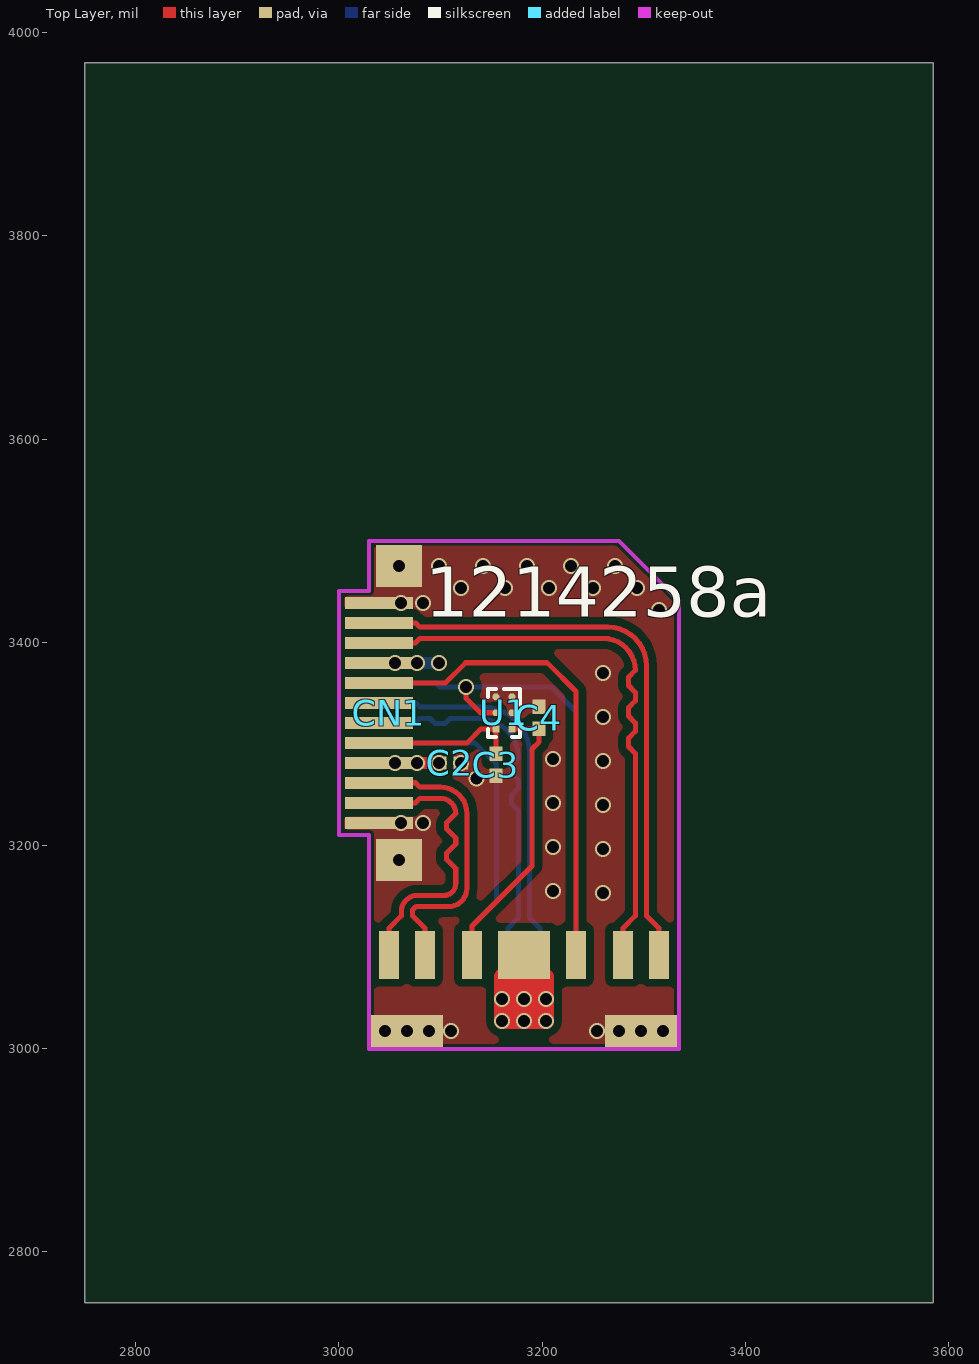
[diagram p0: Top Layer view]
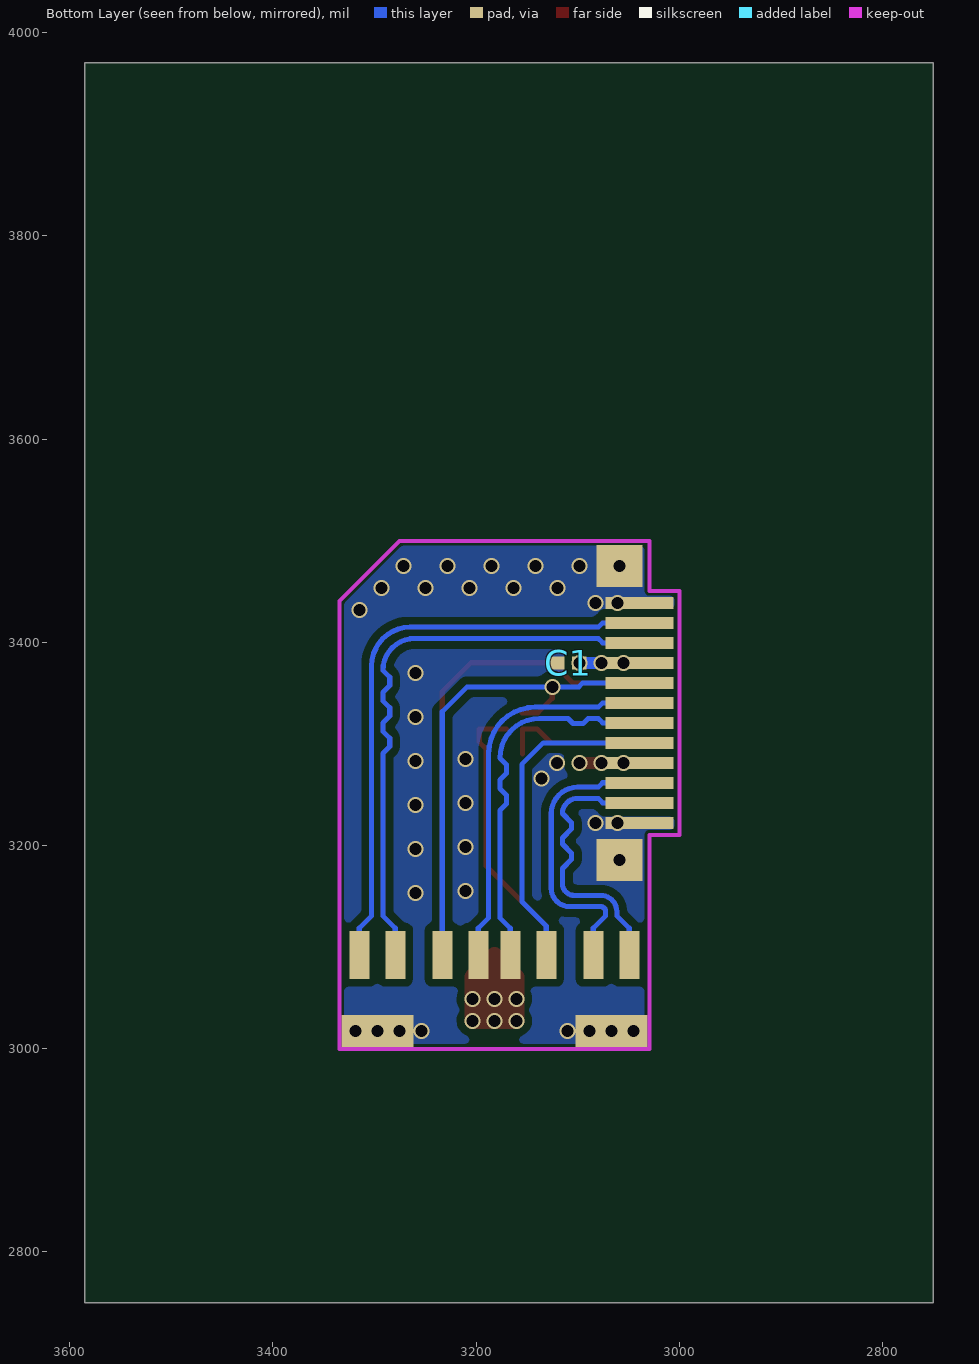
[diagram p1: Bottom Layer view, seen from below]
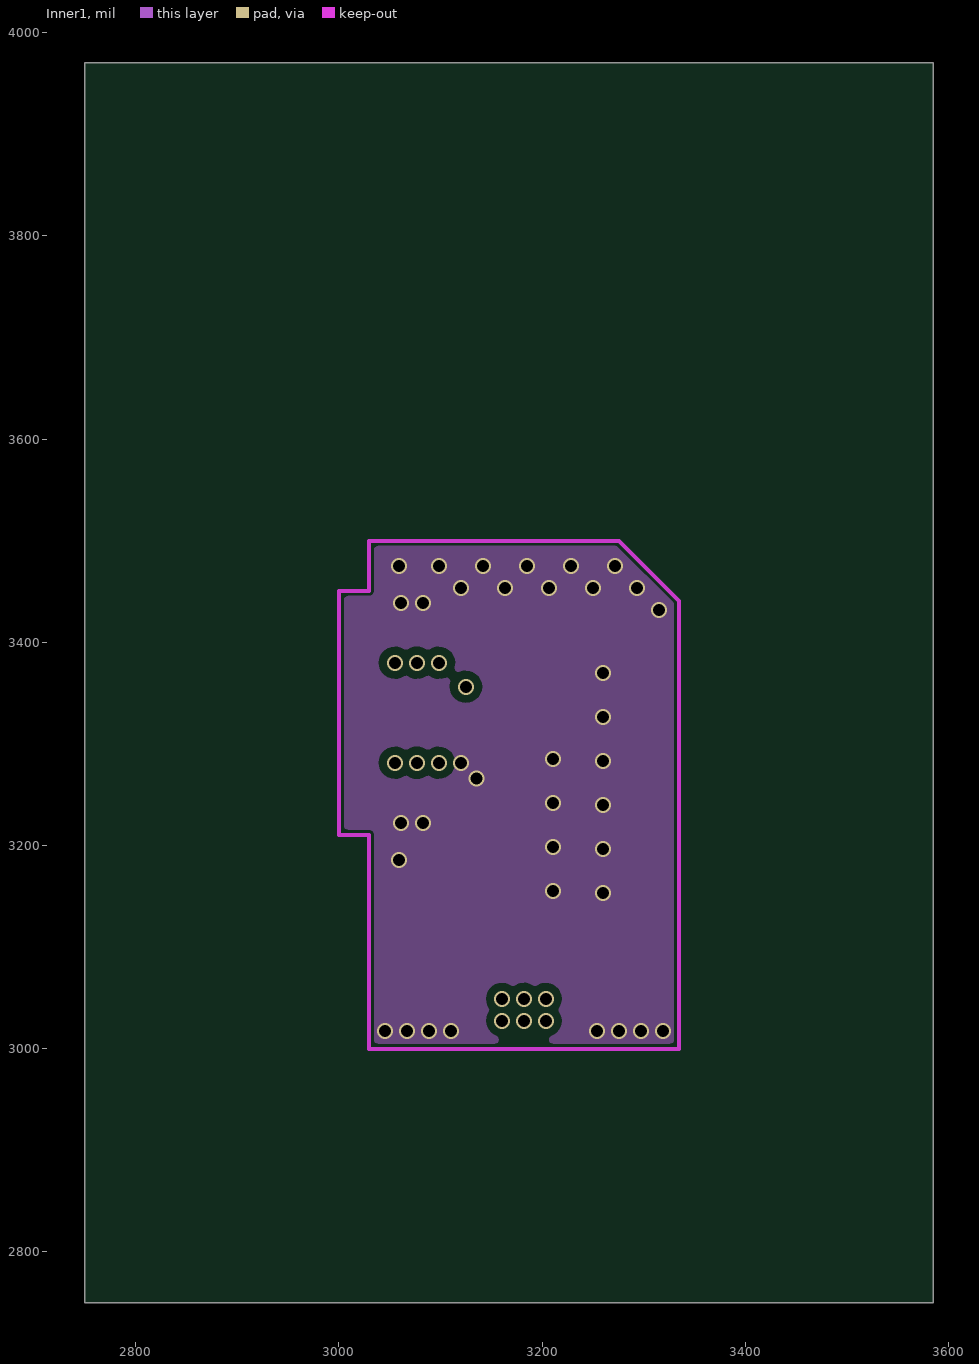
[diagram p2: Inner1]
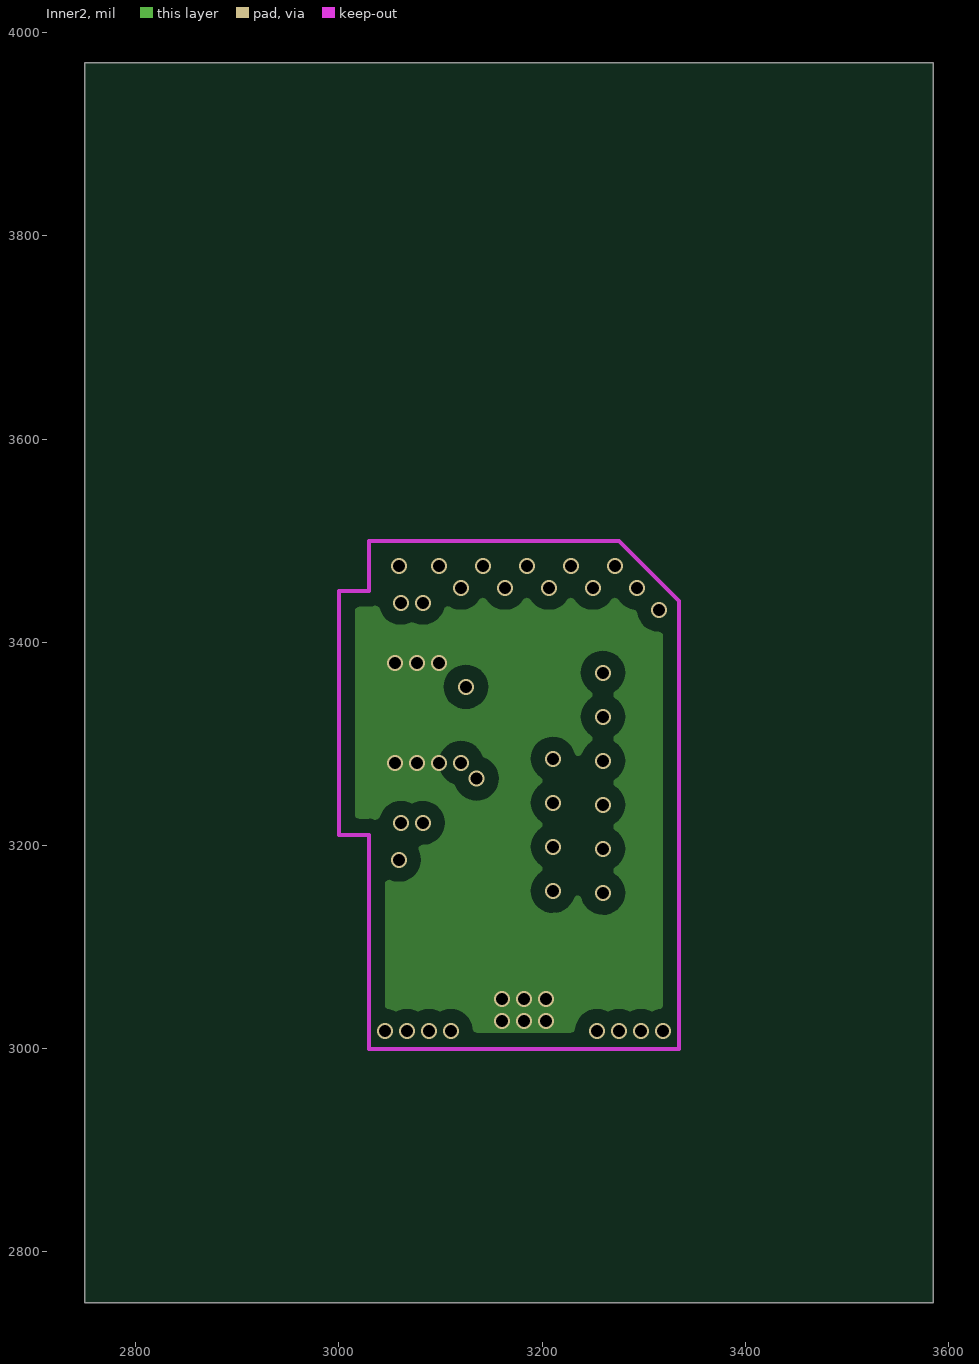
[diagram p3: Inner2]
# Altium PCB MISC82881.pcbdoc
Units mil, origin at the board's own origin, x right, y up, seen from the top; angles counter-clockwise.
Board outline 835 x 1220.35 mil, 4 copper layers (Top Layer, Inner1, Inner2, Bottom Layer), stack 30.706 mil thick; 6 components, 17 nets, 61 pads, 50 vias.

## Layer stack, top to bottom
Top Solder Mask Layer: solder mask 0.394, Dk 0
Top Layer: signal copper 1.378
Dielectric1: surface 8.398, 7628 RC49% 8.6mil, Dk 0
Inner1: signal copper 1.378
Dielectric2: surface 8.398, 1.1mm H/HOZ 含铜, Dk 0
Inner2: signal copper 1.378
Dielectric3: surface 8.398, 7628 RC49% 8.6mil, Dk 0
Bottom Layer: signal copper 1.378
Bottom Solder Mask Layer: solder mask 0.394, Dk 0

## Board outline
3585,2750 2750,2750 2750,3970.35 3585,3970.35

## Design rules (kind name [scope] priority, off if disabled: settings)
BoardOutlineClearance copperThickness2oz_1 [All] p2 off: genericclearance=7.99 ignorepadtopadclearanceinfootprint=FALSE except(0: Arc-SplitContinuation Track-SplitContinuation SMDPad-SplitContinuation THPad-SplitContinuation Via-SplitContinuation Fill-SplitContinuation Region-SplitContinuation Poly-SplitContinuation Text-SplitContinuation Hole-SplitContinuation; 5.98: SMDPad-CutoutEdge THPad-CutoutEdge Via-CutoutEdge Fill-CutoutEdge Region-CutoutEdge Text-CutoutEdge Hole-CutoutEdge; 11.81: Arc-OutlineEdge Track-OutlineEdge SMDPad-OutlineEdge THPad-OutlineEdge Via-OutlineEdge Fill-OutlineEdge Region-OutlineEdge Text-OutlineEdge Hole-OutlineEdge Arc-CutoutEdge Track-CutoutEdge; 13.78: Poly-OutlineEdge Poly-CutoutEdge)
BoardOutlineClearance Plane_innerPlane_1 [All] p4 off: genericclearance=4.02 ignorepadtopadclearanceinfootprint=FALSE except(0: Arc-SplitContinuation Track-SplitContinuation SMDPad-SplitContinuation THPad-SplitContinuation Via-SplitContinuation Fill-SplitContinuation Region-SplitContinuation Poly-SplitContinuation Text-SplitContinuation Hole-SplitContinuation; 5.98: SMDPad-CutoutEdge THPad-CutoutEdge Via-CutoutEdge Fill-CutoutEdge Region-CutoutEdge Text-CutoutEdge Hole-CutoutEdge; 10: Poly-OutlineEdge Poly-CutoutEdge; 11.81: Arc-OutlineEdge Track-OutlineEdge SMDPad-OutlineEdge THPad-OutlineEdge Via-OutlineEdge Fill-OutlineEdge Region-OutlineEdge Text-OutlineEdge Hole-OutlineEdge Arc-CutoutEdge Track-CutoutEdge)
BoardOutlineClearance Copper_copperRegion_1 [All] p6 off: genericclearance=4.02 ignorepadtopadclearanceinfootprint=FALSE except(0: Arc-SplitContinuation Track-SplitContinuation SMDPad-SplitContinuation THPad-SplitContinuation Via-SplitContinuation Fill-SplitContinuation Region-SplitContinuation Poly-SplitContinuation Text-SplitContinuation Hole-SplitContinuation; 5.98: SMDPad-CutoutEdge THPad-CutoutEdge Via-CutoutEdge Fill-CutoutEdge Region-CutoutEdge Text-CutoutEdge Hole-CutoutEdge; 11.81: Arc-OutlineEdge Track-OutlineEdge SMDPad-OutlineEdge THPad-OutlineEdge Via-OutlineEdge Fill-OutlineEdge Region-OutlineEdge Text-OutlineEdge Hole-OutlineEdge Arc-CutoutEdge Track-CutoutEdge; 15.75: Poly-OutlineEdge Poly-CutoutEdge)
BoardOutlineClearance copperThickness1oz_1 [All] p8: genericclearance=4.02 ignorepadtopadclearanceinfootprint=FALSE except(0: Arc-SplitContinuation Track-SplitContinuation SMDPad-SplitContinuation THPad-SplitContinuation Via-SplitContinuation Fill-SplitContinuation Region-SplitContinuation Poly-SplitContinuation Text-SplitContinuation Hole-SplitContinuation; 5.98: SMDPad-CutoutEdge THPad-CutoutEdge Via-CutoutEdge Fill-CutoutEdge Region-CutoutEdge Text-CutoutEdge Hole-CutoutEdge; 11.81: Arc-OutlineEdge Track-OutlineEdge SMDPad-OutlineEdge THPad-OutlineEdge Via-OutlineEdge Fill-OutlineEdge Region-OutlineEdge Text-OutlineEdge Hole-OutlineEdge Arc-CutoutEdge Track-CutoutEdge; 13.78: Poly-OutlineEdge Poly-CutoutEdge)
Clearance copperThickness2oz [All] p1 off: gap=7.99 ignorepadtopadclearanceinfootprint=FALSE except(5.98: SMDPad-Track SMDPad-SMDPad THPad-Track SMDPad-THPad THPad-THPad Track-Via SMDPad-Via THPad-Via Via-Via Fill-Track Region-Track Fill-SMDPad Region-SMDPad Fill-THPad Region-THPad Fill-Via Region-Via Fill-Fill Fill-Region Region-Region Arc-Track Arc-SMDPad Arc-THPad Arc-Via Fill-Arc Region-Arc Arc-Arc Text-Track SMDPad-Text Text-THPad Text-Via Fill-Text Region-Text Arc-Text Text-Text Hole-Track Hole-SMDPad Hole-THPad Hole-Via Fill-Hole Region-Hole Hole-Arc Hole-Text; 13.78: Poly-Track Poly-SMDPad Poly-THPad Poly-Via Poly-Fill Poly-Region Poly-Poly Poly-Arc Poly-Text Poly-Hole)
Clearance Plane_innerPlane [All] p3 off: gap=4.02 ignorepadtopadclearanceinfootprint=FALSE except(5.98: SMDPad-Track SMDPad-SMDPad THPad-Track SMDPad-THPad THPad-THPad Track-Via SMDPad-Via THPad-Via Via-Via Fill-Track Region-Track Fill-SMDPad Region-SMDPad Fill-THPad Region-THPad Fill-Via Region-Via Fill-Fill Fill-Region Region-Region Arc-Track Arc-SMDPad Arc-THPad Arc-Via Fill-Arc Region-Arc Arc-Arc Text-Track SMDPad-Text Text-THPad Text-Via Fill-Text Region-Text Arc-Text Text-Text Hole-Track Hole-SMDPad Hole-THPad Hole-Via Fill-Hole Region-Hole Hole-Arc Hole-Text; 10: Poly-Track Poly-SMDPad Poly-THPad Poly-Via Poly-Fill Poly-Region Poly-Poly Poly-Arc Poly-Text Poly-Hole)
Clearance Copper_copperRegion [All] p5 off: gap=4.02 ignorepadtopadclearanceinfootprint=FALSE except(5.98: SMDPad-Track SMDPad-SMDPad THPad-Track SMDPad-THPad THPad-THPad Track-Via SMDPad-Via THPad-Via Via-Via Fill-Track Region-Track Fill-SMDPad Region-SMDPad Fill-THPad Region-THPad Fill-Via Region-Via Fill-Fill Fill-Region Region-Region Arc-Track Arc-SMDPad Arc-THPad Arc-Via Fill-Arc Region-Arc Arc-Arc Text-Track SMDPad-Text Text-THPad Text-Via Fill-Text Region-Text Arc-Text Text-Text Hole-Track Hole-SMDPad Hole-THPad Hole-Via Fill-Hole Region-Hole Hole-Arc Hole-Text; 13.78: Poly-Track Poly-SMDPad Poly-THPad Poly-Via Poly-Fill Poly-Region Poly-Poly Poly-Arc Poly-Text Poly-Hole)
Clearance copperThickness1oz [All] p7: gap=4.02 ignorepadtopadclearanceinfootprint=FALSE except(5.98: SMDPad-Track SMDPad-SMDPad THPad-Track SMDPad-THPad THPad-THPad Track-Via SMDPad-Via THPad-Via Via-Via Fill-Track Region-Track Fill-SMDPad Region-SMDPad Fill-THPad Region-THPad Fill-Via Region-Via Fill-Fill Fill-Region Region-Region Arc-Track Arc-SMDPad Arc-THPad Arc-Via Fill-Arc Region-Arc Arc-Arc Text-Track SMDPad-Text Text-THPad Text-Via Fill-Text Region-Text Arc-Text Text-Text Hole-Track Hole-SMDPad Hole-THPad Hole-Via Fill-Hole Region-Hole Hole-Arc Hole-Text; 13.78: Poly-Track Poly-SMDPad Poly-THPad Poly-Via Poly-Fill Poly-Region Poly-Poly Poly-Arc Poly-Text Poly-Hole)
DiffPairsRouting differentialPair [All] p1: maxlimit=6 minlimit=6 mostfreqgap=6 toplayer_minwidth=5 toplayer_prefwidth=10 toplayer_maxwidth=100 toplayer_mingap=6 toplayer_prefgap=6 toplayer_maxgap=6 midlayer1_minwidth=5 midlayer1_prefwidth=10 midlayer1_maxwidth=100 midlayer1_mingap=6 midlayer1_prefgap=6 midlayer1_maxgap=6 midlayer2_minwidth=5 midlayer2_prefwidth=10 midlayer2_maxwidth=100 midlayer2_mingap=6 midlayer2_prefgap=6 midlayer2_maxgap=6 bottomlayer_minwidth=5 bottomlayer_prefwidth=10 bottomlayer_maxwidth=100 bottomlayer_mingap=6 bottomlayer_prefgap=6 bottomlayer_maxgap=6 maxuncoupledlength=10
HoleToHoleClearance otherClearance [All] p1: gap=11.8 allowstackedmicrovias=TRUE
Length netLength [All] p1: minlimit=0 maxlimit=0
PasteMaskExpansion pasteMaskExpansion [All] p1: expansion=0
PlaneConnect innerPlane [All] p1: planeconnectstyle=Relief reliefexpansion=20 reliefentries=4 reliefconductorwidth=10 reliefairgap=10
PolygonConnect copperRegion [All] p1: connectstyle=Direct reliefconductorwidth=10 reliefentries=4 polygonreliefangle="90 Angle" airgapwidth=10 via.connectstyle=Relief via.reliefconductorwidth=10 via.reliefentries=4 via.polygonreliefangle="90 Angle" via.airgapwidth=10
RoutingVias viaSize [All] p1: holewidth=12.01 width=24.02 viastyle="Through Hole" minholewidth=11.81 minwidth=19.68 maxholewidth=248.03 maxwidth=393.7
SolderMaskExpansion solderMaskExpansion [IsVia] p1: expansion=-1000 istentingtop=TRUE
SolderMaskExpansion solderMaskExpansion [All] p2: expansion=2.01 istentingtop=FALSE
Width copperThickness2oz_2 [All] p1 off: maxlimit=100 minlimit=8 preferedwidth=10
Width copperThickness1oz_2 [All] p2: maxlimit=100 minlimit=5 preferedwidth=10

## Components (designator, comment, footprint, x,y, rotation, side; value= is the part's Value field where it differs from the comment)
C1 "" c0201 3098.43,3379.92 r0 bottom
C2 "" c0201 3098.43,3281.5 r0 top
C3 "" c0201 3154.5,3290.38 r270 top
C4 "" c0201 3196.85,3314.96 r90 top
CN1 "" 简易版公头 3000,3330.71 r90 top
U1 "" wlcsp-6_l1.2-w0.8-r2-c3-p0.40-tl改 3162.4,3330.71 r270 top

## Footprints (in the part's own frame and the unit in brackets; to place one, negate y for a bottom-side part, rotate by r counter-clockwise, add the part's x,y. Pads: shape width x height; smd on the part's side, far side on the other; paste and mask are expansions set on the pad)
c0201 [mil]
  rect 14.51x12.76 smd paste-3937.01 mask+2: 1(0,0) 2(21.6,0)
wlcsp-6_l1.2-w0.8-r2-c3-p0.40-tl改 [mm]
  round 0.174 smd paste+0 mask+0.025: A1(-0.4,0.201) A2(-0.4,-0.201) B1(-0.001,0.201) B2(-0.001,-0.198)
  rect 0.174x0.174 smd paste+0 mask+0.025: C1(0.4,0.201) C2(0.4,-0.201)
  silkscreen extent -0.6,-0.4 0.6,0.4
简易版公头 [mm]
  rect 0.3x1.7 smd far side paste+0 mask+0.051: A1(2.75,-1) A2(2.25,-1) A3(1.75,-1) A4(1.25,-1) A5(0.75,-1) A6(0.25,-1) A7(-0.25,-1) A8(-0.75,-1) A9(-1.25,-1) A10(-1.75,-1) A11(-2.25,-1) A12(-2.75,-1)
  rect 1.05x1.15 smd far side paste+0 mask+0.025: A1(3.675,-1.5) A12(-3.675,-1.5)
  rect 1.05x1.15 smd paste+0 mask+0.025: B1(-3.675,-1.5) B12(3.675,-1.5)
  rect 0.3x1.7 smd paste+0 mask+0.05: B1(-2.75,-1) B2(-2.25,-1) B3(-1.75,-1) B4(-1.25,-1) B5(-0.75,-1) B6(-0.25,-1) B7(0.25,-1) B8(0.75,-1) B9(1.25,-1) B10(1.75,-1) B11(2.25,-1) B12(2.75,-1)
  Board Outline Layer lines w0.1: -4.3,-0.75 -3.05,-0.75 -3.05,0 3.05,0 3.05,-0.75 4.3,-0.75

## Free pads (board coordinates)
  rect 19.68x47.24 smd far side paste-3937.01 mask+1.97: 7(3049.21,3092.52) 7(3084.65,3092.52) 7(3130.91,3092.52) 7(3166.34,3092.52) 7(3197.83,3092.52) 7(3233.27,3092.52) 7(3279.53,3092.52) 7(3314.96,3092.52)
  rect 19.68x47.24 smd paste-3937.01 mask+1.97: 7(3049.21,3092.52) 7(3084.65,3092.52) 7(3130.91,3092.52) 7(3233.27,3092.52) 7(3279.53,3092.52) 7(3314.96,3092.52)
  rect 70.87x31.5 smd far side paste-3937.01 mask+1.97: 7(3066.93,3017.72) 7(3297.24,3017.72)
  rect 70.87x31.5 smd paste-3937.01 mask+1.97: 7(3066.93,3017.72) 7(3297.24,3017.72)
  rect 51.18x47.24 smd paste-3937.01 mask+1.97: 7(3182.09,3092.52)

## Via types
v1: diameter 15.75, hole 11.8, Top Layer to Bottom Layer, 50 vias

## Nets (pads, with @x,y where several pads share a name; then routed paths per layer and width w, separated by ;. In a path a pad name is that pad's centre, name@x,y a point inside that pad or via, vN(x,y) a via of type N, cw(c..) or ccw(c..) an arc to the next point about the centre after c; other vN are vias at no path point)
CC: CN1.A5 pad.7@3233.27,3092.52 U1.B2 | length 491.7
  Top Layer w5: v1(3125,3356.3) 3125,3345 3139.24,3330.76 U1.B2
  Bottom Layer w5: CN1.A5 3095,3360.24 3098.94,3356.3 v1(3125,3356.3) 3208.7,3356.3 3233.27,3331.73 pad.7@3233.27,3092.52
D+: CN1.A6 pad.7@3197.83,3092.52 | length 378.4
  Bottom Layer w5: CN1.A6 3075.32,3340.55 3079.67,3336.21 3142.06,3336.21 cw(c3142.06,3290.68) 3187.59,3290.68 3187.59,3128.89 3197.83,3118.64 pad.7@3197.83,3092.52
D-: CN1.A7 pad.7@3166.34,3092.52 | length 374.2
  Bottom Layer w5: CN1.A7 3075.32,3320.87 3079.67,3325.21 3089.61,3325.21 3094.61,3320.21 3104.61,3320.21 3109.61,3325.21 3137.5,3325.21 cw(c3137.5,3286.12) 3176.59,3286.12 3170,3279.54 3170,3271.12 3176.59,3264.54 3176.59,3256.12 3170,3249.54 3170,3241.12 3176.59,3234.54 3176.59,3128.89 3166.34,3118.64 pad.7@3166.34,3092.52
GND: C1.2 C2.2 C3.2 C4.2 CN1.A1 CN1.A12 CN1.B1 CN1.B12 pad.7@3066.93,3017.72 pad.7@3297.24,3017.72 U1.A1 U1.A2 U1.B1
  other v1: 3045.28,3017.72 3066.93,3017.72 3088.58,3017.72 3110.23,3017.72 3253.94,3017.72 3275.59,3017.72 3297.24,3017.72 3318.9,3017.72 3259.84,3153.57 3210.63,3155.52 3059.06,3186.03 3259.84,3196.87 3210.63,3198.83 3061.03,3222.44 3082.68,3222.44 3259.84,3240.17 3210.63,3242.13 3135.46,3266.05 3120.15,3281.36 3259.84,3283.47 3210.63,3285.43 3259.84,3326.78 3259.84,3370.08 3314.94,3432.09 3061.01,3438.98 3082.66,3438.98 3120.08,3453.74 3163.38,3453.74 3206.68,3453.74 3249.98,3453.74 3293.29,3453.74 3059.06,3475.39 3098.43,3475.39 3141.73,3475.39 3185.03,3475.39 3228.33,3475.39 3271.64,3475.39
RX1+: CN1.B11 pad.7@3314.96,3092.52 | length 576.4
  Top Layer w5: CN1.B11 3075.32,3419.29 3079.67,3414.95 3264.85,3414.95 cw(c3264.85,3377.06) 3302.74,3377.06 3302.74,3130.86 3314.96,3118.64 pad.7@3314.96,3092.52
RX1-: CN1.B10 pad.7@3279.53,3092.52 | length 573.9
  Top Layer w5: CN1.B10 3075.32,3399.61 3079.67,3403.95 3260.29,3403.95 cw(c3260.29,3372.5) 3291.74,3372.5 3285,3365.76 3285,3357.5 3291.74,3350.76 3291.74,3342.5 3285,3335.76 3285,3327.5 3291.74,3320.76 3291.74,3312.5 3285,3305.76 3285,3297.5 3291.74,3290.76 3291.74,3130.86 3279.53,3118.64 pad.7@3279.53,3092.52
RX2+: CN1.A11 pad.7@3049.21,3092.52 | length 286.7
  Bottom Layer w5: CN1.A11 3075.32,3242.13 3079.67,3246.48 3100,3246.48 cw(c3100,3231.48) 3115,3231.48 3106,3222.48 3106,3216.48 3115,3207.48 3115,3201.48 3106,3192.48 3106,3186.48 3115,3177.48 3115,3162.5 cw(c3103.5,3162.5) 3103.5,3151 3077.43,3151 ccw(c3077.43,3135) 3061.43,3135 3061.43,3130.86 3049.21,3118.64 pad.7@3049.21,3092.52
RX2-: CN1.A10 pad.7@3084.65,3092.52 | length 291
  Bottom Layer w5: CN1.A10 3075.32,3261.83 3079.67,3257.48 3100,3257.48 cw(c3100,3231.48) 3126,3231.48 3126,3157.94 cw(c3108.06,3157.94) 3108.06,3140 3077.43,3140 ccw(c3077.43,3135) 3072.43,3135 3072.43,3130.86 3084.65,3118.64 pad.7@3084.65,3092.52
SBU1: CN1.A8 pad.7@3130.91,3092.52 | length 321.9
  Bottom Layer w5: CN1.A8 3133.82,3301.18 3155,3280 3155,3145 3130.91,3120.91 pad.7@3130.91,3092.52
SBU2: CN1.B8 pad.7@3233.27,3092.52 | length 473
  Top Layer w5: CN1.B8 3105,3360.23 3124.77,3380 3205,3380 3233.27,3351.73 pad.7@3233.27,3092.52
TX1+: CN1.A2 pad.7@3314.96,3092.52 | length 576.4
  Bottom Layer w5: CN1.A2 3075.32,3419.29 3079.67,3414.95 3264.85,3414.95 cw(c3264.85,3377.06) 3302.74,3377.06 3302.74,3130.86 3314.96,3118.64 pad.7@3314.96,3092.52
TX1-: CN1.A3 pad.7@3279.53,3092.52 | length 573.9
  Bottom Layer w5: CN1.A3 3075.32,3399.61 3079.67,3403.95 3260.29,3403.95 cw(c3260.29,3372.5) 3291.74,3372.5 3285,3365.76 3285,3357.5 3291.74,3350.76 3291.74,3342.5 3285,3335.76 3285,3327.5 3291.74,3320.76 3291.74,3312.5 3285,3305.76 3285,3297.5 3291.74,3290.76 3291.74,3130.86 3279.53,3118.64 pad.7@3279.53,3092.52
TX2+: CN1.B2 pad.7@3049.21,3092.52 | length 286.7
  Top Layer w5: CN1.B2 3075.32,3242.13 3079.67,3246.48 3100,3246.48 cw(c3100,3231.48) 3115,3231.48 3106,3222.48 3106,3216.48 3115,3207.48 3115,3201.48 3106,3192.48 3106,3186.48 3115,3177.48 3115,3162.5 cw(c3103.5,3162.5) 3103.5,3151 3077.43,3151 ccw(c3077.43,3135) 3061.43,3135 3061.43,3130.86 3049.21,3118.64 pad.7@3049.21,3092.52
TX2-: CN1.B3 pad.7@3084.65,3092.52 | length 291
  Top Layer w5: CN1.B3 3075.32,3261.83 3079.67,3257.48 3100,3257.48 cw(c3100,3231.48) 3126,3231.48 3126,3157.94 cw(c3108.06,3157.94) 3108.06,3140 3077.43,3140 ccw(c3077.43,3135) 3072.43,3135 3072.43,3130.86 3084.65,3118.64 pad.7@3084.65,3092.52
VBUS: C1.1 C2.1 CN1.A4 CN1.A9 CN1.B4 CN1.B9 pad.7@3182.09,3092.52 | length 309.3
  Top Layer w11.81: CN1.B4 v1(3055.12,3281.5) v1(3076.77,3281.5) v1(3098.42,3281.5)
  Top Layer w15.75: v1(3160.44,3027.57) v1(3160.44,3049.22) 3160.44,3070.87 3182.09,3092.52 3203.74,3070.87 v1(3203.74,3049.22) v1(3203.74,3027.57) v1(3182.09,3027.57) v1(3160.44,3027.57)
  Bottom Layer w11.81: CN1.A4 v1(3055.12,3379.92) v1(3076.77,3379.92) v1(3098.42,3379.92)
  other v1: 3182.09,3049.22
VCONN1: C3.1 CN1.B5 U1.C2 | length 145.4
  Top Layer w5: CN1.B5 3126.18,3301.18 3139.96,3314.96 U1.C2 C3.1
VCONN2: C4.1 pad.7@3130.91,3092.52 U1.C1 | length 276.3
  Top Layer w5: pad.7@3130.91,3092.52 3130.91,3120.91 3190,3180 3190,3295 3196.85,3301.85 3196.85,3314.96 U1.C1
pads on no net: CN1.B6 CN1.B7

## Polygon pours and split planes (outlines as drawn)
GND on Bottom Layer (solid, remove dead copper, pour order 2): 3029.53,3500 3029.53,3450.79 3000,3450.79 3000,3210.63 3029.53,3210.63 3029.53,3000 3334.65,3000 3335,3000.36 3335,3440 3275.59,3499.41 3275.59,3500
GND on Inner1 (solid, remove dead copper): 3029.53,3500 3029.53,3450.79 3000,3450.79 3000,3210.63 3029.53,3210.63 3029.53,3000 3334.65,3000 3335,3000.36 3335,3440 3275.59,3499.41 3275.59,3500
GND on Top Layer (solid, remove dead copper, pour order 4): 3029.53,3500 3029.53,3450.79 3000,3450.79 3000,3210.63 3029.53,3210.63 3029.53,3000 3334.65,3000 3335,3000.36 3335,3440 3275.59,3499.41 3275.59,3500
VBUS on Inner2 (solid, remove dead copper): 3029.53,3500 3029.53,3450.79 3000,3450.79 3000,3210.63 3029.53,3210.63 3029.53,3000 3334.65,3000 3335,3000.36 3335,3440 3275.59,3499.41 3275.59,3500

## Keep-outs
Board Outline Layer:
  lines w3.94: 3029.53,3161.42 3029.53,3000 3334.65,3000 3334.65,3440.94 3275.59,3500 3029.53,3500

## Other copper
Top Layer:
  region net VBUS: 3182.09,3092.52 3160.44,3070.87 3160.44,3027.57 3203.74,3027.57 3203.74,3070.87

## Silkscreen, mask and mechanical layers (free items; w line width, h text height)
Top Silkscreen Layer:
  text "1214258a" at 3085,3425 h49.21